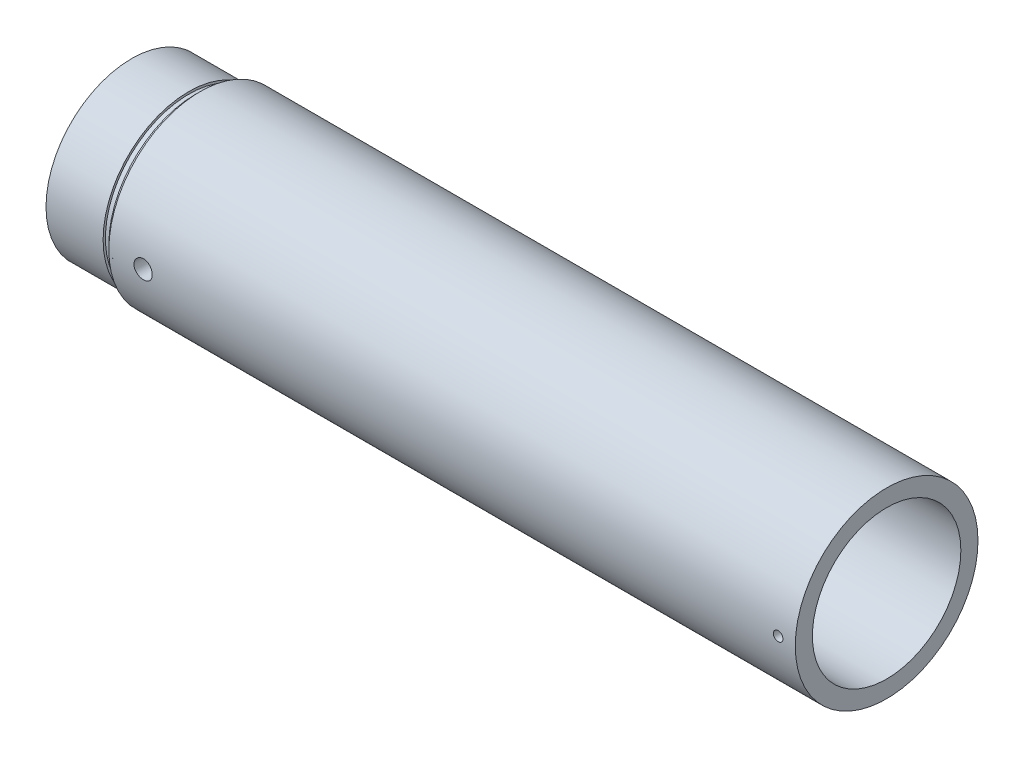
from build123d import *

# Parameters (mm, degrees)
SKETCH2_R               = 32.5
CUT_EXTRUDE1_DEPTH      = 50
SKETCH3_R               = 30
CUT_EXTRUDE2_DEPTH      = 287.147252302
CHAMFER1_SIZE           = 1.5
CHAMFER2_SIZE           = 1.5
CUT_EXTRUDE3_DEPTH      = 336.306203343
CUT_EXTRUDE3_DEPTH_BACK = 336.306203343
SKETCH4_R               = 4
SKETCH7_W               = 2.1
SKETCH7_H               = 40


with BuildPart() as part:
    # Sketch1 → Revolve1 (revolve)
    with BuildSketch(Plane.XY, mode=Mode.PRIVATE) as revolve1_sk:
        Polygon((0, 0), (0, 37.5), (25, 37.5), (25, 36.5), (28, 36.5), (28, 38), (30, 38), (30, 40), (330.5, 40), (330.5, 0), align=None)
    revolve(revolve1_sk.sketch.rotate(Axis((0, 0, 0), (-1, 0, 0)), 90), axis=Axis((0, 0, 0), (-1, 0, 0)))

    # Sketch2 → Cut-Extrude1 (cut)
    with BuildSketch(Plane(origin=(330.5, 0, 0), x_dir=(0, 0, -1), z_dir=(1, 0, 0))):
        Circle(SKETCH2_R)
    extrude(amount=-CUT_EXTRUDE1_DEPTH, mode=Mode.SUBTRACT)

    # Sketch3 → Cut-Extrude2 (cut, through all)
    with BuildSketch(Plane(origin=(280.5, 0, 0), x_dir=(0, 0, -1), z_dir=(1, 0, 0))):
        Circle(SKETCH3_R)
    extrude(amount=-CUT_EXTRUDE2_DEPTH, mode=Mode.SUBTRACT)

    # Chamfer1
    chamfer1_edges = [part.edges().sort_by_distance(p)[0] for p in [
        (280.5, 0, 32.5),
    ]]
    chamfer(chamfer1_edges, length=CHAMFER1_SIZE)

    # Chamfer2
    chamfer2_edges = [part.edges().sort_by_distance(p)[0] for p in [
        (0, 0, 30),
    ]]
    chamfer(chamfer2_edges, length=CHAMFER2_SIZE)

    # Sketch4 → Cut-Extrude3 (cut, two sides: drawn at the far end of the back side and taken through both)
    with BuildSketch(Plane.XY.offset(-CUT_EXTRUDE3_DEPTH_BACK)):
        with Locations((45, 0)):
            Circle(SKETCH4_R)
    extrude(amount=CUT_EXTRUDE3_DEPTH + CUT_EXTRUDE3_DEPTH_BACK, mode=Mode.SUBTRACT)

    # Sketch7 → M5 Tapped Hole2 (revolve, cut)
    with BuildSketch(Plane.YZ.offset(323)):
        with Locations((1.05, 20)):
            Rectangle(SKETCH7_W, SKETCH7_H)
    revolve(axis=Axis((323, 0, -6.35), (0, 0, 1)), mode=Mode.SUBTRACT)


solid = part.part
